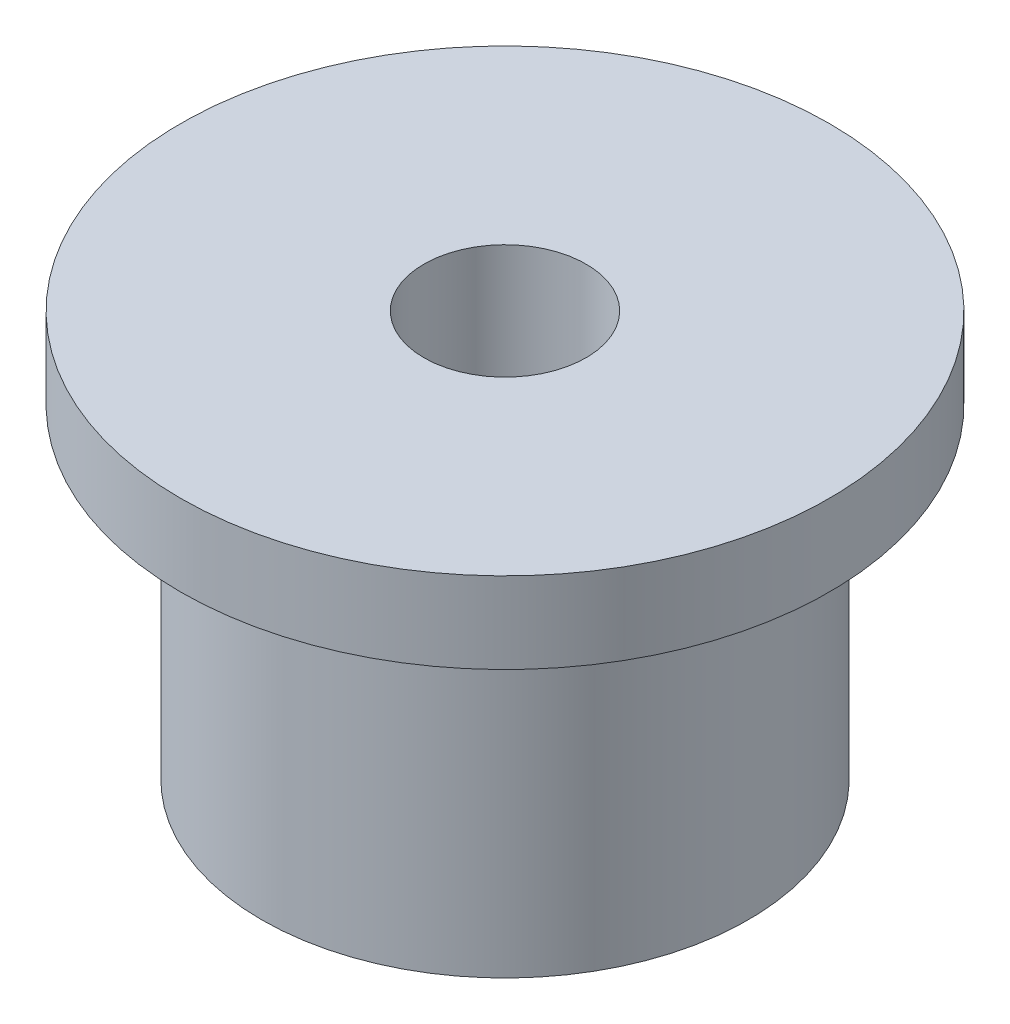
SolidWorks part; units mm, degrees
ref_plane "Front Plane" through (0, 0, 0) normal (0, 0, 1) x (1, 0, 0)
ref_plane "Top Plane" through (0, 0, 0) normal (0, 1, 0) x (1, 0, 0)
ref_plane "Right Plane" through (0, 0, 0) normal (1, 0, 0) x (0, 0, -1)
sketch "Sketch1" plane through (0, 0, 0) normal (0, 0, 1) x (1, 0, 0)
  line L0 (0, 71.0883) -> (0, -192.8339) construction
  line L1 (-25, 0) -> (-100, 0)
  line L2 (-100, 0) -> (-100, -25)
  line L3 (-100, -25) -> (-75, -25)
  line L4 (-75, -25) -> (-75, -125)
  line L5 (-75, -125) -> (-25, -125)
  line L6 (-25, -125) -> (-25, 0)
  dimension "D1" = 25
  dimension "D2" = 75
  dimension "D3" = 100
  dimension "D4" = 125
  dimension "D5" = 25
revolve "Revolve1" add sketch "Sketch1" angle 360 about L0
